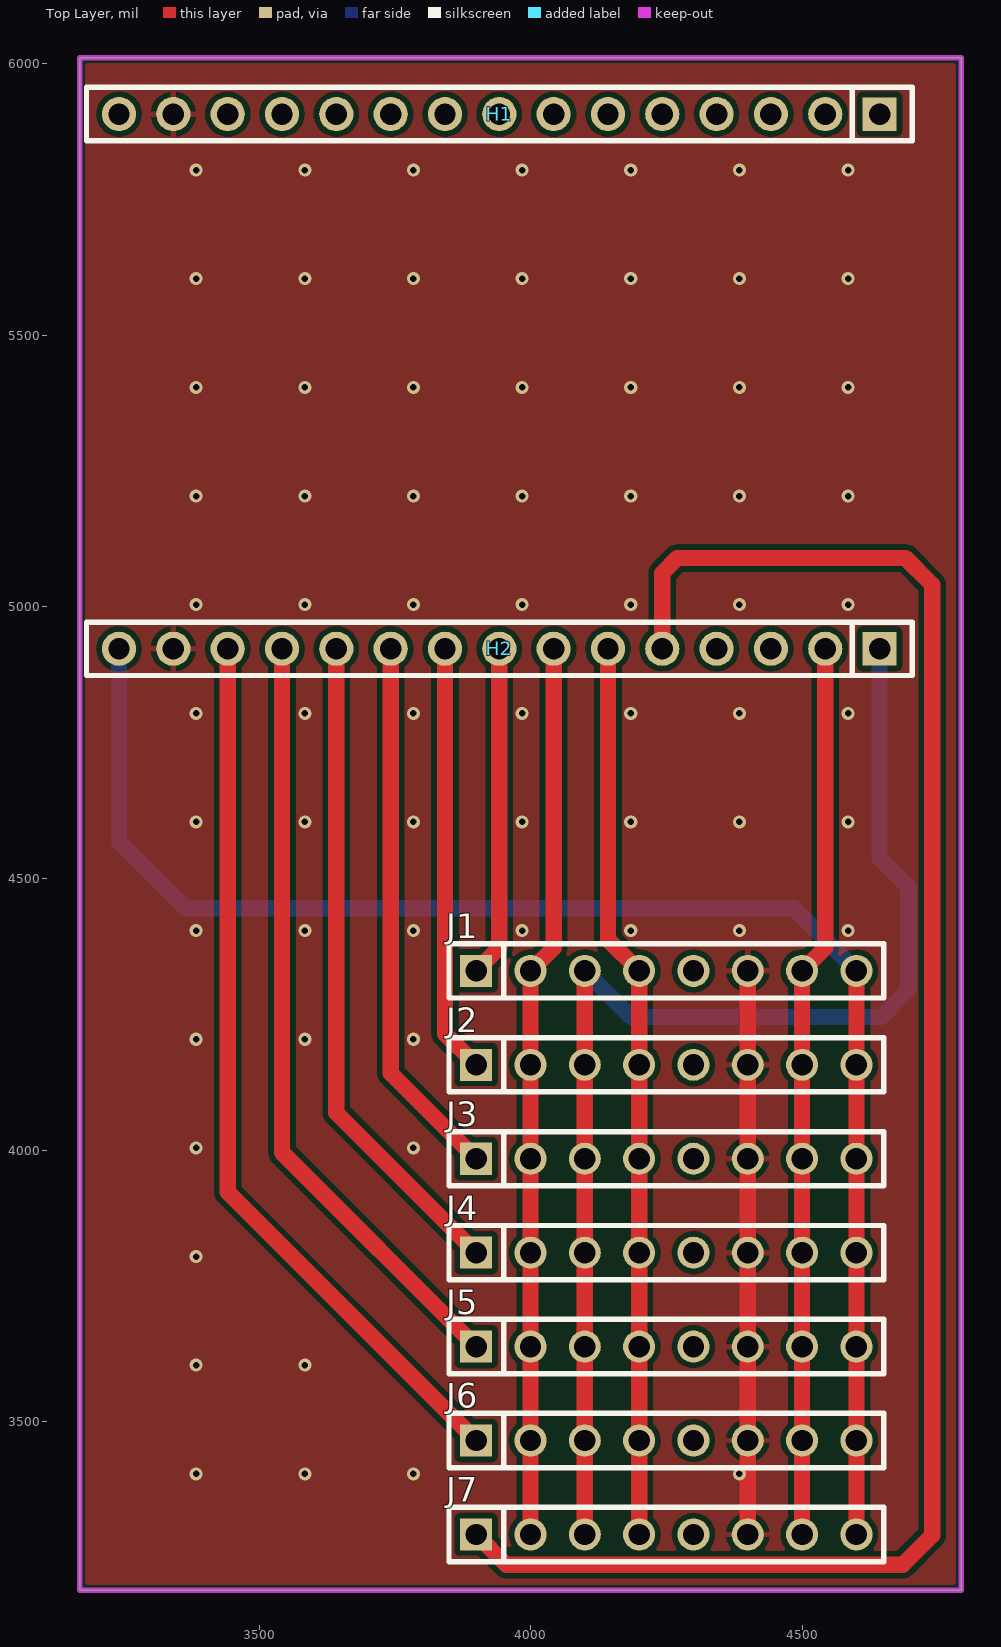
[diagram p0: Top Layer view]
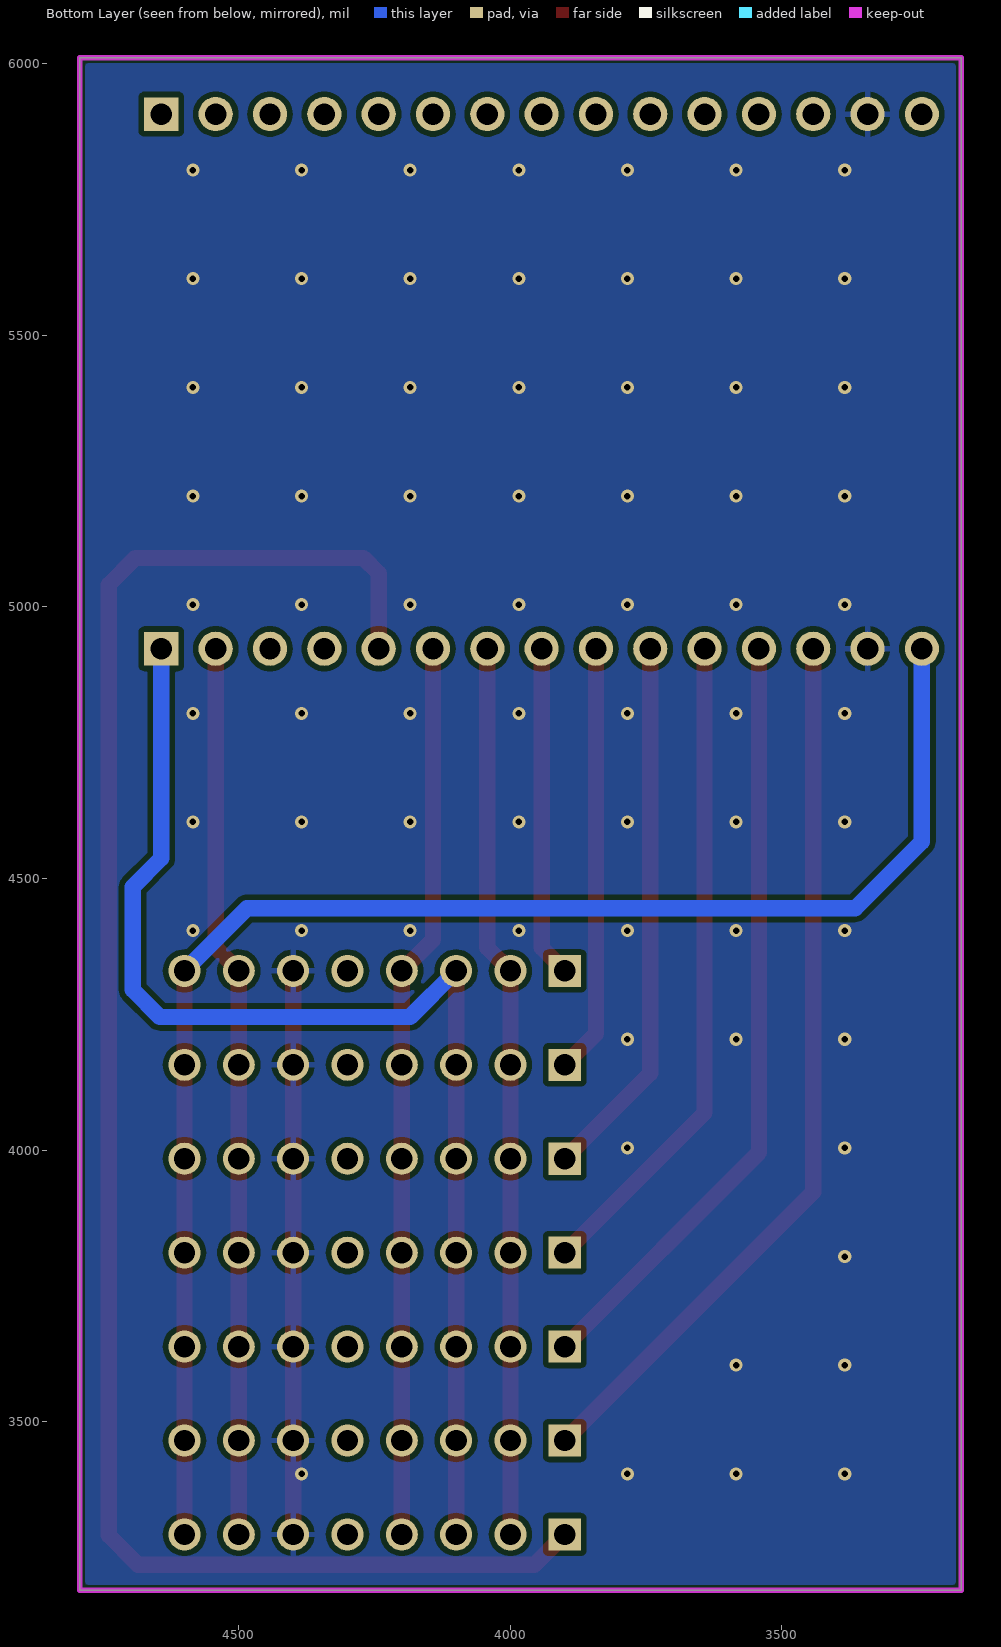
[diagram p1: Bottom Layer view, seen from below]
# Altium PCB MISC49852.pcbdoc
Units mil, origin at the board's own origin, x right, y up, seen from the top; angles counter-clockwise.
Board outline 1622.17 x 2820.67 mil, 2 copper layers (Top Layer, Bottom Layer), stack 62.206 mil thick; 9 components, 13 nets, 86 pads, 68 vias.

## Layer stack, top to bottom
Top Solder Mask Layer: solder mask 0.394, Dk 3.3
Top Layer: signal copper 1.379
Dielectric1: surface 59.449, FR4, Dk 4.5
Bottom Layer: signal copper 1.378
Bottom Solder Mask Layer: solder mask 0.394, Dk 3.3

## Board outline
3170,6010.67 3170,3190 4792.17,3190 4792.17,6010.67

## Design rules (kind name [scope] priority, off if disabled: settings)
BoardOutlineClearance copperThickness2oz_1 [All] p2 off: genericclearance=7.99 ignorepadtopadclearanceinfootprint=FALSE except(0: Arc-SplitContinuation Track-SplitContinuation SMDPad-SplitContinuation THPad-SplitContinuation Via-SplitContinuation Fill-SplitContinuation Region-SplitContinuation Poly-SplitContinuation Text-SplitContinuation Hole-SplitContinuation; 5.98: Arc-CutoutEdge SMDPad-CutoutEdge THPad-CutoutEdge Via-CutoutEdge Fill-CutoutEdge Region-CutoutEdge Text-CutoutEdge; 6.93: Hole-OutlineEdge Hole-CutoutEdge; 10: Poly-OutlineEdge Poly-CutoutEdge; 11.81: Arc-OutlineEdge Track-OutlineEdge SMDPad-OutlineEdge THPad-OutlineEdge Via-OutlineEdge Fill-OutlineEdge Region-OutlineEdge Text-OutlineEdge Track-CutoutEdge)
BoardOutlineClearance copperThickness1oz_1 [All] p4: genericclearance=4.02 ignorepadtopadclearanceinfootprint=FALSE except(0: Arc-SplitContinuation Track-SplitContinuation SMDPad-SplitContinuation THPad-SplitContinuation Via-SplitContinuation Fill-SplitContinuation Region-SplitContinuation Poly-SplitContinuation Text-SplitContinuation Hole-SplitContinuation; 6: SMDPad-CutoutEdge THPad-CutoutEdge Via-CutoutEdge Fill-CutoutEdge Region-CutoutEdge Text-CutoutEdge; 6.93: Hole-OutlineEdge Hole-CutoutEdge; 10: Poly-OutlineEdge Poly-CutoutEdge; 11.8: Arc-OutlineEdge Track-OutlineEdge SMDPad-OutlineEdge THPad-OutlineEdge Via-OutlineEdge Fill-OutlineEdge Region-OutlineEdge Text-OutlineEdge; 11.81: Arc-CutoutEdge Track-CutoutEdge)
Clearance copperThickness2oz [All] p1 off: gap=7.99 ignorepadtopadclearanceinfootprint=FALSE except(5.98: SMDPad-Track SMDPad-SMDPad THPad-Track SMDPad-THPad THPad-THPad Track-Via SMDPad-Via THPad-Via Via-Via Fill-Track Region-Track Fill-SMDPad Region-SMDPad Fill-THPad Region-THPad Fill-Via Region-Via Fill-Fill Fill-Region Region-Region Arc-Track Arc-SMDPad Arc-THPad Arc-Via Fill-Arc Region-Arc Arc-Arc Text-Track SMDPad-Text Text-THPad Text-Via Fill-Text Region-Text Arc-Text Text-Text; 6.93: Hole-Track Hole-SMDPad Hole-THPad Hole-Via Fill-Hole Region-Hole Hole-Arc Hole-Text; 10: Poly-Track Poly-SMDPad Poly-THPad Poly-Via Poly-Fill Poly-Region Poly-Poly Poly-Arc Poly-Text Poly-Hole)
Clearance copperThickness1oz [All] p3: gap=4.02 ignorepadtopadclearanceinfootprint=FALSE except(5.98: SMDPad-Track SMDPad-SMDPad THPad-Track SMDPad-THPad THPad-THPad Track-Via SMDPad-Via THPad-Via Via-Via Fill-Track Region-Track Fill-SMDPad Region-SMDPad Fill-THPad Region-THPad Fill-Via Region-Via Fill-Fill Fill-Region Region-Region; 6: Arc-Track Arc-SMDPad Arc-THPad Arc-Via Fill-Arc Region-Arc Arc-Arc Text-Track SMDPad-Text Text-THPad Text-Via Fill-Text Region-Text Arc-Text Text-Text; 6.93: Hole-Track Hole-SMDPad Hole-THPad Hole-Via Fill-Hole Region-Hole Hole-Arc Hole-Text; 10: Poly-Track Poly-SMDPad Poly-THPad Poly-Via Poly-Fill Poly-Region Poly-Poly Poly-Arc Poly-Text Poly-Hole)
DiffPairsRouting differentialPair [All] p1: maxlimit=6 minlimit=6 mostfreqgap=6 toplayer_minwidth=5 toplayer_prefwidth=10 toplayer_maxwidth=100 toplayer_mingap=6 toplayer_prefgap=6 toplayer_maxgap=6 bottomlayer_minwidth=5 bottomlayer_prefwidth=10 bottomlayer_maxwidth=100 bottomlayer_mingap=6 bottomlayer_prefgap=6 bottomlayer_maxgap=6 maxuncoupledlength=10
HoleToHoleClearance otherClearance [All] p1: gap=11.81 allowstackedmicrovias=TRUE
Length netLength [All] p1: minlimit=0 maxlimit=0
MatchedLengths netLengthTolerance [All] p1: tolerance=1000
PasteMaskExpansion pasteMaskExpansion [All] p1: expansion=0
PlaneConnect innerPlane [All] p1: planeconnectstyle=Relief reliefexpansion=20 reliefentries=4 reliefconductorwidth=10 reliefairgap=10
PolygonConnect copperRegion [(InNet('GND'))] p1: connectstyle=Relief reliefconductorwidth=10 reliefentries=4 polygonreliefangle="90 Angle" airgapwidth=10 via.connectstyle=Relief via.reliefconductorwidth=10 via.reliefentries=4 via.polygonreliefangle="90 Angle" via.airgapwidth=10
RoutingVias viaSize [All] p1: holewidth=12.01 width=24.02 viastyle="Through Hole" minholewidth=11.81 minwidth=19.68 maxholewidth=248.03 maxwidth=393.7
SolderMaskExpansion solderMaskExpansion [IsVia] p1: expansion=-1000 istentingtop=TRUE
SolderMaskExpansion solderMaskExpansion [All] p2: expansion=2 istentingtop=FALSE
Width copperThickness2oz_2 [All] p1 off: maxlimit=100 minlimit=8 preferedwidth=10
Width copperThickness1oz_2 [All] p2: maxlimit=100 minlimit=5 preferedwidth=10

## Components (designator, comment, footprint, x,y, rotation, side; value= is the part's Value field where it differs from the comment)
H1 "" HDR-TH_15P-P2.54-V-F-1 3942.13,5907.13 r180 top
H2 "" HDR-TH_15P-P2.54-V-F-1 3942.13,4922.87 r180 top
J1 "" HDR-TH_8P-P2.54-V-M 4249.52,4330 r0 top
J2 "" HDR-TH_8P-P2.54-V-M 4249.52,4157.08 r0 top
J3 "" HDR-TH_8P-P2.54-V-M 4249.52,3984.17 r0 top
J4 "" HDR-TH_8P-P2.54-V-M 4249.52,3811.25 r0 top
J5 "" HDR-TH_8P-P2.54-V-M 4249.52,3638.33 r0 top
J6 "" HDR-TH_8P-P2.54-V-M 4249.52,3465.42 r0 top
J7 "" HDR-TH_8P-P2.54-V-M 4249.52,3292.5 r0 top

## Footprints (in the part's own frame and the unit in brackets; to place one, negate y for a bottom-side part, rotate by r counter-clockwise, add the part's x,y. Pads: shape width x height; smd on the part's side, far side on the other; paste and mask are expansions set on the pad)
HDR-TH_8P-P2.54-V-M [mm]
  rect 1.5x1.5 hole 1: 1(-8.89,0)
  round 1.5 hole 1: 2(-6.35,0) 3(-3.81,0) 4(-1.27,0) 5(1.27,0) 6(3.81,0) 7(6.35,0) 8(8.89,0)
  silkscreen extent -10.16,-1.27 10.16,1.27
HDR-TH_15P-P2.54-V-F-1 [mm]
  rect 1.6x1.575 hole 1: 1(-17.78,0)
  round 1.6 hole 1: 2(-15.24,0) 3(-12.7,0) 4(-10.16,0) 5(-7.62,0) 6(-5.08,0) 7(-2.54,0) 8(0,0) 9(2.54,0) 10(5.08,0) 11(7.62,0) 12(10.16,0) 13(12.7,0) 14(15.24,0) 15(17.78,0)
  silkscreen extent -19.3,-1.25 19.3,1.25

## Via types
v1: diameter 24.02, hole 12, Top Layer to Bottom Layer, 68 vias

## Nets (pads, with @x,y where several pads share a name; then routed paths per layer and width w, separated by ;. In a path a pad name is that pad's centre, name@x,y a point inside that pad or via, vN(x,y) a via of type N, cw(c..) or ccw(c..) an arc to the next point about the centre after c; other vN are vias at no path point)
2: H2.12 J5.1 | length 1432.6
  Top Layer w30: H2.12 3542.13,3995.73 J5.1
4: H2.11 J4.1 | length 1218.2
  Top Layer w30: H2.11 3642.13,4068.65 J4.1
5: H2.8 J1.1 | length 610.5
  Top Layer w30: J1.1 3942.13,4372.6 H2.8
15: H2.13 J6.1 | length 1646.9
  Top Layer w30: H2.13 3442.13,3922.82 J6.1
16: H2.10 J3.1 | length 1003.9
  Top Layer w30: H2.10 3742.13,4141.57 J3.1
17: H2.9 J2.1 | length 789.6
  Top Layer w30: H2.9 3842.13,4214.48 J2.1
18: H2.7 J1.2 J2.2 J3.2 J4.2 J5.2 J6.2 J7.2 | length 1648
  Top Layer w30: J7.2 J6.2 J5.2 J4.2 J3.2 J2.2 J1.2 4042.13,4372.6 H2.7
19: H2.6 J1.4 J2.4 J3.4 J4.4 J5.4 J6.4 J7.4 | length 1654.1
  Top Layer w30: H2.6 4142.13,4387.4 J1.4 J2.4 J3.4 J4.4 J5.4 J6.4 J7.4
21: H2.5 J7.1 | length 3303.2
  Top Layer w30: J7.1 3955.22,3236.8 4685,3236.8 4739.1,3290.9 4739.1,5040.9 4690,5090 4270,5090 4242.13,5062.13 H2.5
22: H2.2 J1.7 J2.7 J3.7 J4.7 J5.7 J6.7 J7.7 | length 1648
  Top Layer w30: J7.7 J6.7 J5.7 J4.7 J3.7 J2.7 J1.7 4542.13,4372.6 H2.2
23: H2.1 J1.3 J2.3 J3.3 J4.3 J5.3 J6.3 J7.3 | length 2338.7
  Top Layer w30: J7.3 J6.3 J5.3 J4.3 J3.3 J2.3 J1.3
  Bottom Layer w30: J1.3 4184.52,4245 4645,4245 4695,4295 4695,4484.25 4642.13,4537.13 H2.1
GND: H1.14 H2.14 J1.6 J2.6 J3.6 J4.6 J5.6 J6.6 J7.6 | length 1037.5
  Top Layer w30: J7.6 J6.6 J5.6 J4.6 J3.6 J2.6 J1.6
  other v1: 3384.1,3404.1 3584.1,3404.1 3784.1,3404.1 4384.1,3404.1 3384.1,3604.1 3584.1,3604.1 3384.1,3804.1 3384.1,4004.1 3784.1,4004.1 3384.1,4204.1 3584.1,4204.1 3784.1,4204.1 3384.1,4404.1 3584.1,4404.1 3784.1,4404.1 3984.1,4404.1 4184.1,4404.1 4384.1,4404.1 4584.1,4404.1 3384.1,4604.1 3584.1,4604.1 3784.1,4604.1 3984.1,4604.1 4184.1,4604.1 4384.1,4604.1 4584.1,4604.1 3384.1,4804.1 3584.1,4804.1 3784.1,4804.1 3984.1,4804.1 4184.1,4804.1 4384.1,4804.1 4584.1,4804.1 3384.1,5004.1 3584.1,5004.1 3784.1,5004.1 3984.1,5004.1 4184.1,5004.1 4384.1,5004.1 4584.1,5004.1 3384.1,5204.1 3584.1,5204.1 3784.1,5204.1 3984.1,5204.1 4184.1,5204.1 4384.1,5204.1 4584.1,5204.1 3384.1,5404.1 3584.1,5404.1 3784.1,5404.1 3984.1,5404.1 4184.1,5404.1 4384.1,5404.1 4584.1,5404.1 3384.1,5604.1 3584.1,5604.1 3784.1,5604.1 3984.1,5604.1 4184.1,5604.1 4384.1,5604.1 4584.1,5604.1 3384.1,5804.1 3584.1,5804.1 3784.1,5804.1 3984.1,5804.1 4184.1,5804.1 4384.1,5804.1 4584.1,5804.1
VCC: H2.15 J1.8 J2.8 J3.8 J4.8 J5.8 J6.8 J7.8 | length 2848.4
  Top Layer w30: J7.8 J6.8 J5.8 J4.8 J3.8 J2.8 J1.8
  Bottom Layer w30: H2.15 3242.13,4567.87 3365,4445 4484.52,4445 J1.8
pads on no net: H1.1 H1.2 H1.3 H1.4 H1.5 H1.6 H1.7 H1.8 H1.9 H1.10 H1.11 H1.12 H1.13 H1.15 H2.3 H2.4 J1.5 J2.5 J3.5 J4.5 J5.5 J6.5 J7.5

## Polygon pours and split planes (outlines as drawn)
GND on Bottom Layer (solid, remove dead copper, pour order 2): 3015,6085 3015,3000 5040,3000 5040,6085
GND on Top Layer (solid, remove dead copper, pour order 0): 3000,6130 3000,3085 5325,3085 5325,6130

## Keep-outs
Board Outline Layer:
  the board outline again, w10